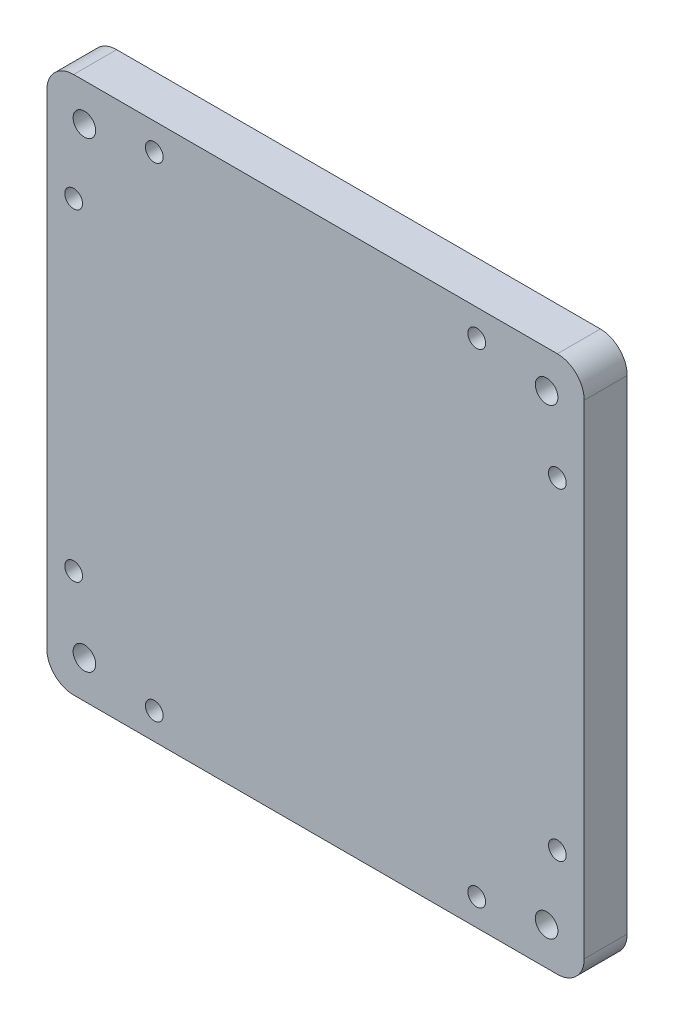
from build123d import *

# Parameters (mm, degrees)
BOSS_EXTRUDE1_DEPTH   = 8
M5_TAPPED_HOLE1_D     = 4.2
M5_TAPPED_HOLE1_DEPTH = 12.4
M5_TAPPED_HOLE1_TIP   = 1.2618073
M4_TAPPED_HOLE1_D     = 3.3
M4_TAPPED_HOLE1_DEPTH = 10.1
M4_TAPPED_HOLE1_TIP   = 0.991420021


with BuildPart() as part:
    # Sketch1 → Boss-Extrude1 (new body)
    with BuildSketch(Plane.XY):
        with BuildLine():
            Line((-45, 50), (45, 50))
            ThreePointArc((45, 50), (48.535533906, 48.535533906), (50, 45))
            Line((50, 45), (50, -45))
            ThreePointArc((50, -45), (48.535533906, -48.535533906), (45, -50))
            Line((45, -50), (-45, -50))
            ThreePointArc((-45, -50), (-48.535533906, -48.535533906), (-50, -45))
            Line((-50, -45), (-50, 45))
            ThreePointArc((-50, 45), (-48.535533906, 48.535533906), (-45, 50))
        make_face()
    extrude(amount=BOSS_EXTRUDE1_DEPTH)

    # M5 Tapped Hole1
    with Locations(Plane(origin=(-43, 43, 8), x_dir=(1, 0, 0), z_dir=(0, 0, 1))):
        with Locations((0, 0), (86, 0), (86, -86), (0, -86)):
            Hole(M5_TAPPED_HOLE1_D / 2, depth=M5_TAPPED_HOLE1_DEPTH)
            with Locations((0, 0, -(M5_TAPPED_HOLE1_DEPTH + M5_TAPPED_HOLE1_TIP / 2))):  # 118° drill point
                Cone(0, M5_TAPPED_HOLE1_D / 2, M5_TAPPED_HOLE1_TIP, mode=Mode.SUBTRACT)

    # M4 Tapped Hole1
    with Locations(Plane(origin=(-30, -45, 8), x_dir=(1, 0, 0), z_dir=(0, 0, 1))):
        with Locations((0, 0), (60, 0), (-15, 15), (-15, 75), (75, 75), (75, 15), (0, 90), (60, 90)):
            Hole(M4_TAPPED_HOLE1_D / 2, depth=M4_TAPPED_HOLE1_DEPTH)
            with Locations((0, 0, -(M4_TAPPED_HOLE1_DEPTH + M4_TAPPED_HOLE1_TIP / 2))):  # 118° drill point
                Cone(0, M4_TAPPED_HOLE1_D / 2, M4_TAPPED_HOLE1_TIP, mode=Mode.SUBTRACT)


solid = part.part
